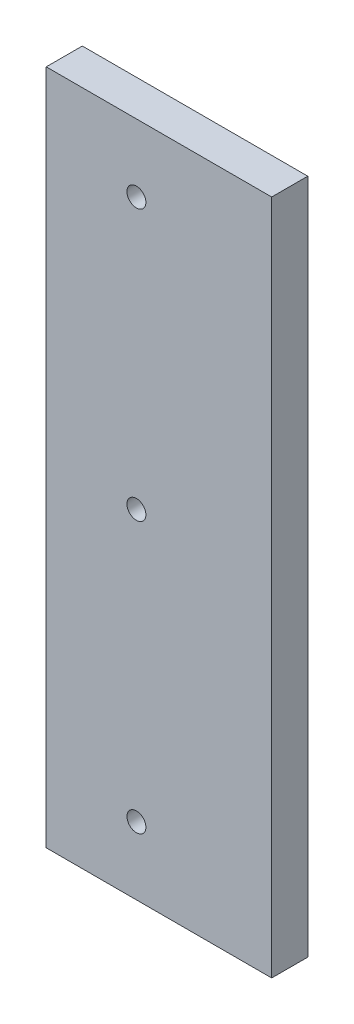
from build123d import *

# Parameters (mm, degrees)
SKETCH1_W           = 50
SKETCH1_H           = 150
BOSS_EXTRUDE1_DEPTH = 4
M5_TAPPED_HOLE1_D   = 4.2


with BuildPart() as part:
    # Sketch1 → Boss-Extrude1 (new, symmetric)
    with BuildSketch(Plane.XY):
        Rectangle(SKETCH1_W, SKETCH1_H)
    extrude(amount=BOSS_EXTRUDE1_DEPTH, both=True)

    # M5 Tapped Hole1 (through all)
    with Locations(Plane.XY.offset(4)):
        with Locations((-5, 60), (-5, -60), (-5, 0)):
            Hole(M5_TAPPED_HOLE1_D / 2)


solid = part.part
